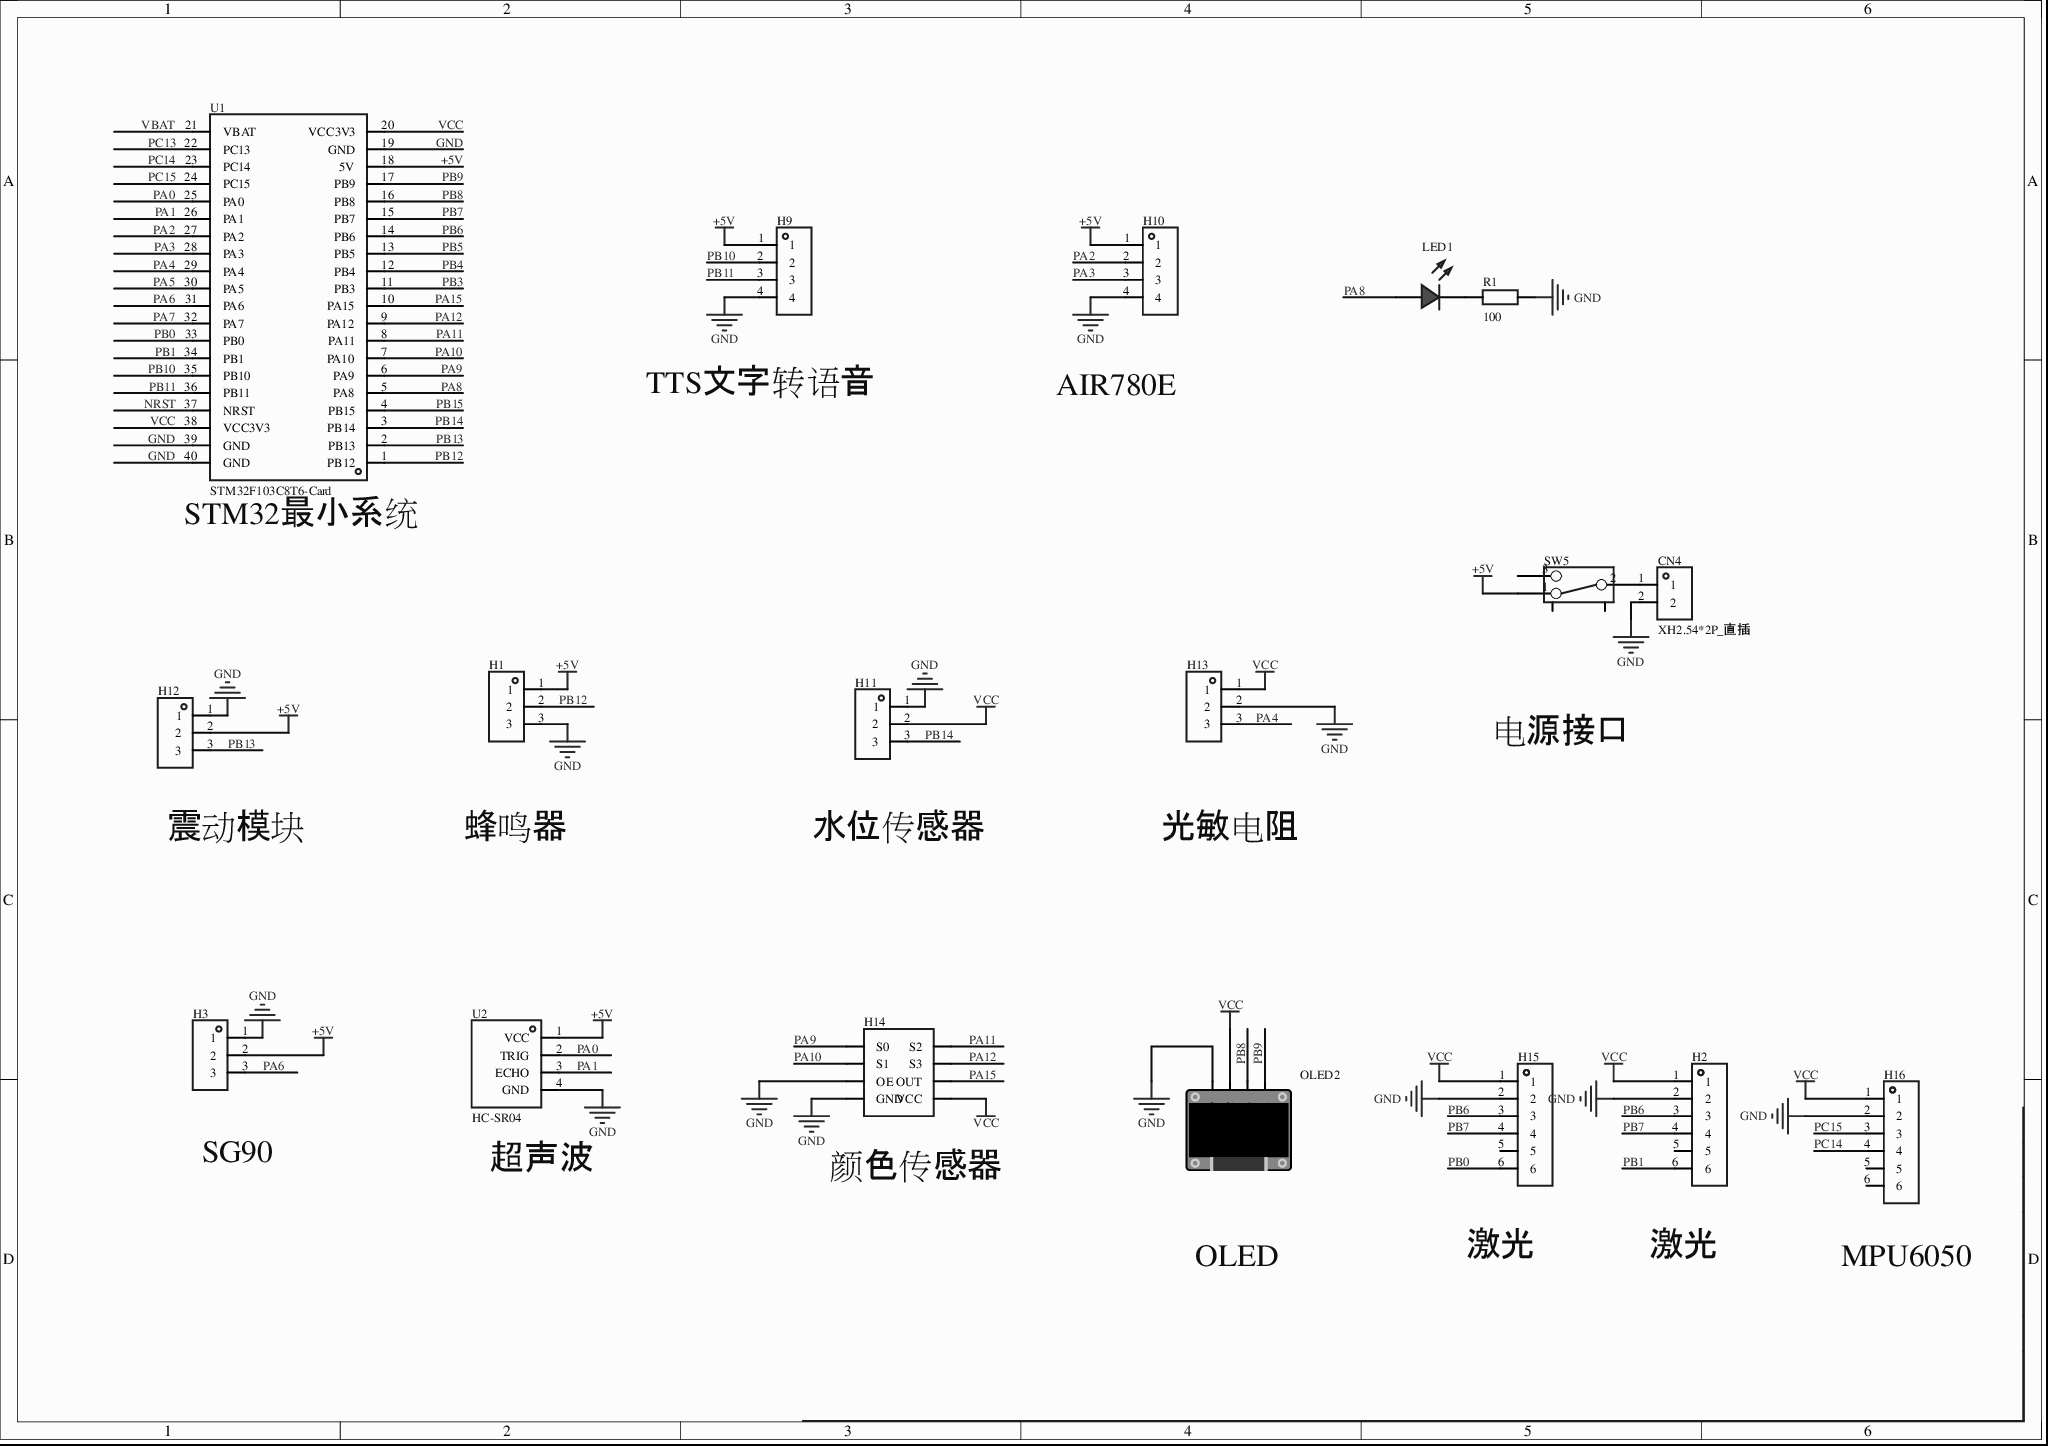
[diagram p0: MISC51292-3.schdoc]
# Altium project MISC51292-2.PrjPcb
1 sheet, 18 parts. Net scope: global (net labels, ports and power ports of the same name join across sheets).
Board file: MISC51292.pcbdoc

## Sheet MISC51292-3.schdoc
size 297 x 209 mm; Version: V1.0; @Project Name: MISC51292; @Page Count: 1; @Update Date: 2026-04-28; @Create Date: 2026-04-28; @Schematic Name: MISC51292; @Page No: 1; @Create Time: 23:22:16; @Update Time: 17:32:40; @Board Name: MISC51292

### Parts
CN4  XH2.54*2P_直插  [CONN-TH_2P-P2.50-XH2.54-2P]
H1  (no value)  [HDR-TH_3P-P2.54-V-F]
H2  (no value)  [HDR-TH_6P-P2.54-V-F]
H3  (no value)  [HDR-TH_3P-P2.54-V-M]
H9  (no value)  [HDR-TH_4P-P2.54-V-M]
H10  (no value)  [HDR-TH_4P-P2.54-V-M]
H11  (no value)  [HDR-TH_3P-P2.54-V-F]
H12  (no value)  [HDR-TH_3P-P2.54-V-F]
H13  (no value)  [HDR-TH_3P-P2.54-V-F]
H14  (no value)  [HDR-TH_8P-P2.54-V-F-R2-C4-S2.54-1]
H15  (no value)  [HDR-TH_6P-P2.54-V-F]
H16  (no value)  [HDR-TH_6P-P2.54-V-F]
LED1  (no value)  [LED_TH-3mm]
OLED2  (no value)  [0.96OLED_4P]
R1  100  [Res_1/8W]
SW5  (no value)  [拨动开关]
U1  STM32F103C8T6-Card  [CONN-TH_L53.3-W22.9_STM32F103C8T6-CARD]
U2  HC-SR04  [TH_HC-SR04V]

### Nets
+5V: H1.1 H3.2 H9.1 H10.1 H12.2 SW5.1 U1.18(5V) U2.1(VCC)
GND: CN4.2 H1.3 H2.2 H3.1 H9.4 H10.4 H11.1 H12.1 H13.2 H14.5(OE) H14.7(GND) H15.2 H16.2 OLED2.1(GND) R1.2 U1.19(GND) U1.39(GND) U1.40(GND) U2.4(GND)
VCC: H2.1 H11.2 H13.1 H14.8(VCC) H15.1 H16.1 OLED2.2(VCC) U1.20(VCC3V3) U1.38(VCC3V3)
NRST: U1.37(NRST)
PA0: U1.25(PA0) U2.2(TRIG)
PA1: U1.26(PA1) U2.3(ECHO)
PA2: H10.2 U1.27(PA2)
PA3: H10.3 U1.28(PA3)
PA4: H13.3 U1.29(PA4)
PA5: U1.30(PA5)
PA6: H3.3 U1.31(PA6)
PA7: U1.32(PA7)
PA8: LED1.1(C) U1.5(PA8)
PA9: H14.1(S0) U1.6(PA9)
PA10: H14.3(S1) U1.7(PA10)
PA11: H14.2(S2) U1.8(PA11)
PA12: H14.4(S3) U1.9(PA12)
PA15: H14.6(OUT) U1.10(PA15)
PB0: H15.6 U1.33(PB0)
PB1: H2.6 U1.34(PB1)
PB3: U1.11(PB3)
PB4: U1.12(PB4)
PB5: U1.13(PB5)
PB6: H2.3 H15.3 U1.14(PB6)
PB7: H2.4 H15.4 U1.15(PB7)
PB8: OLED2.3(SCL) U1.16(PB8)
PB9: OLED2.4(SDA) U1.17(PB9)
PB10: H9.2 U1.35(PB10)
PB11: H9.3 U1.36(PB11)
PB12: H1.2 U1.1(PB12)
PB13: H12.3 U1.2(PB13)
PB14: H11.3 U1.3(PB14)
PB15: U1.4(PB15)
PC13: U1.22(PC13)
PC14: H16.4 U1.23(PC14)
PC15: H16.3 U1.24(PC15)
VBAT: U1.21(VBAT)
NetCN4_1: CN4.1 SW5.2
NetLED1_2: LED1.2(A) R1.1

Not connected (* = marked no-connect by the designer): H2 5; H15 5; H16 5 6; SW5 3 4 5

### Notes on the sheet
- 串口：
  TTS文字转语音模块  		PB10，PB11
  AIR780E 4G模块            PA2.PA3
  GPIO:
  LED灯	PA8
  震动模块PB13
  蜂鸣器  PB12
  水位传感器：PB14
  光敏电阻模块 （DO）PA4
  SG90舵机 PA6
  HCSR04超声波模块 TRIG PA0  ECHO PA1
  TCS3200颜色识别 S1-S4 PA9-PA12 OUT-PA15
  IIC:
  0.96英寸OLED显示屏	PB8，PB9
  VL53L0X激光模块（两个） PB6 PB7  XSHUT1 PB0 XSHUT2 PB1
  MPU6050 SCL PC15  SDA PC14
- TTS文字转语音
- AIR780E
- (near U1) STM32最小系统
- 电源接口
- (near H12) 震动模块
- 蜂鸣器
- 水位传感器
- 光敏电阻
- (near H3) SG90
- (near U2) 超声波
- (near H14) 颜色传感器
- OLED
- (near H15) 激光
- (near H2) 激光
- (near H16) MPU6050

### Library data of the parts
CN4 = XH2.54*2P_直插: 3D Model: 325c595e30db4df8abe76612dd40b0fa0819f05c4eef4c71ace90d822a990e87; 3D Model Transform: 295.275,228.346,0,180,0,0,-0.002,-20.079,-137.795; AddInBom: yes; Device: XH2.54*2P_直插; Symbol: XH2.54*2P_直插; LCSC Part Name: XH2.54*2P_直插; Supplier Part: C9900008615; Manufacturer Part: XH2.54*2P_直插; Supplier Footprint: XH2.54_2P; JLCPCB Part Class: Extended Part; Supplier: LCSC; FootprintName: CONN-TH_2P-P2.50-XH2.54-2P; ConvertToPcb: yes; ModelName: CONN-TH_2P-P2.50-XH2.54-2P
H1 H11-H13 = HDR-F_2.54_1x3P: Symbol: PM254V-11-03-H85; 3D Model: f3b3cc5aae9641bf9e56fc160cef875b; 3D Model Transform: 299.9994,100,0,0,0,0,0,0,-118.11; ConvertToPcb: yes; ModelName: HDR2.54-F-LI-1X3P; Device: HDR-F_2.54_1x3P; Supplier Part: C541850; Supplier Footprint: 插件; FootprintName: HDR-TH_3P-P2.54-V-F; AddInBom: yes
H2 H15 H16 = HDR-F_2.54_1x6P: Symbol: Header-Female-2.54_1x6; 3D Model: 0f5bcf94dcda47d085f24cdca1696fe9; 3D Model Transform: 619.684,94.488,0,0,0,0,0,0,-125.984; ConvertToPcb: yes; Device: HDR-F_2.54_1x6P; Supplier Part: C40877; Supplier Footprint: 插件; AddInBom: yes; FootprintName: HDR-TH_6P-P2.54-V-F; ModelName: HDR-TH_6P-P2.54-V-F
H3 = HDR-M_2.54_1x3P: AddInBom: yes; ModelId: bb473b6d38ff42a99216a4fcdbdcc4cb0819f05c4eef4c71ace90d822a990e87; ModelName: HDR-TH_3P-P2.54-M-LI-1X3P; ModelTransform: 300.03877,100,0,0,0,0,0,0,-118.11; Symbol: HDR-M_2.54_1x3P; Device: HDR-M_2.54_1x3P; ConvertToPcb: yes; FootprintName: HDR-TH_3P-P2.54-V-M; SupplierPart: C2937625; Supplier Footprint: 插件
H9 H10 = HDR-M_2.54_1x4P: Symbol: PZ254V-11-04P; ConvertToPcb: yes; ModelId: 112f4d05e8d64e99ab9a333894bea4f90819f05c4eef4c71ace90d822a990e87; ModelName: HDR-TH_4P-P2.54-M-LI-1X4P; ModelTransform: 399.999,104.7242,0,0,0,0,0,0,-118.11; Device: HDR-M_2.54_1x4P; AddInBom: yes; SupplierPart: C492403; Supplier Footprint: 插件; FootprintName: HDR-TH_4P-P2.54-V-M
H14 = HDR-F_2.54_2x4: Symbol: HDR-F-2.54_2x4; ConvertToPcb: yes; ModelId: 64729f32a5874cf59655d275a66f10500819f05c4eef4c71ace90d822a990e87; ModelName: HDR2.54-F-LI-2X4P; ModelTransform: 399.999,200,0,0,0,0,0,0,-118.11; Device: HDR-F_2.54_2x4; AddInBom: yes; SupplierPart: C92271; Supplier Footprint: 插件; FootprintName: HDR-TH_8P-P2.54-V-F-R2-C4-S2.54-1
LED1 = LED_TH-R_3mm: 3D Model: a497c992633541038a38947cdc58012f0819f05c4eef4c71ace90d822a990e87; 3D Model Transform: 141.274,153.327,0,0,0,0,-5.984,0,-137.795; ConvertToPcb: yes; ModelName: LED-TH-3mm_R; Symbol: LED_TH-R; Device: LED_TH-R_3mm; Supplier Footprint: 插件; AddInBom: yes; FootprintName: LED_TH-3mm
OLED2 = 0.96OLED模块_4P: 3D Model: 79c000fdb68d45a296c2e9bedf4f9055; 3D Model Transform: 1393.69792,1318.895,0,0,0,0,0,-560.079,-137.795; ConvertToPcb: yes; Symbol: 0.96OLED模块_4P; Device: 0.96OLED模块_4P; Supplier Footprint: 插件; AddInBom: yes; FootprintName: 0.96OLED_4P; ModelName: 0.96OLED_4P
R1 = Res_AXIAL-1/8W: Symbol: 电阻; 3D Model: b2b5ae7ae4c642178fe0039925c86a3f0819f05c4eef4c71ace90d822a990e87; 3D Model Transform: 282.86,66.88,253.09,0,0,0,0,0,-191; ConvertToPcb: yes; ModelName: RES-TH_BD1.8-L3.2-P7.20-D0.4; Device: Res_AXIAL-1/8W; Value: 100; Supplier Footprint: 轴向引线; AddInBom: yes; FootprintName: Res_1/8W
SW5 = 拨动开关_正: 3D Model: 4321fe59a4074cbfb4989553f297c68f0819f05c4eef4c71ace90d822a990e87; 3D Model Transform: 370.09,208.7,472.35,0,0,0,0,0,-110; ConvertToPcb: yes; ModelName: SW-TH_SS-12D02-VG4; Device: 拨动开关_正; Symbol: 拨动开关; Supplier Footprint: 插件; FootprintName: 拨动开关; AddInBom: yes
U1 = STM32F103C8T6-Card: AddInBom: yes; Device: STM32F103C8T6-Card; Symbol: STM32F103C8T6-CARD; LCSC Part Name: STM32F103C8T6-Card; Supplier Part: C9900077949; Manufacturer Part: STM32F103C8T6-Card; Supplier Footprint: 插件; Supplier: LCSC; FootprintName: CONN-TH_L53.3-W22.9_STM32F103C8T6-CARD; ConvertToPcb: yes
U2 = HC-SR04: Manufacturer: Universal Microelectronics; AddInBom: yes; Symbol: HC-SR04; Device: HC-SR04; LCSC Part Name: HC-SR04; SupplierPart: C19857336; ManufacturerPart: HC-SR04; Supplier Footprint: -; JLCPCB Part Class: 扩展库; Datasheet: https://atta.szlcsc.com/upload/public/pdf/source/20240122/47B8E374E428935B7962A2189EF91AAC.pdf; Supplier: LCSC; ConvertToPcb: yes; FootprintName: TH_HC-SR04V